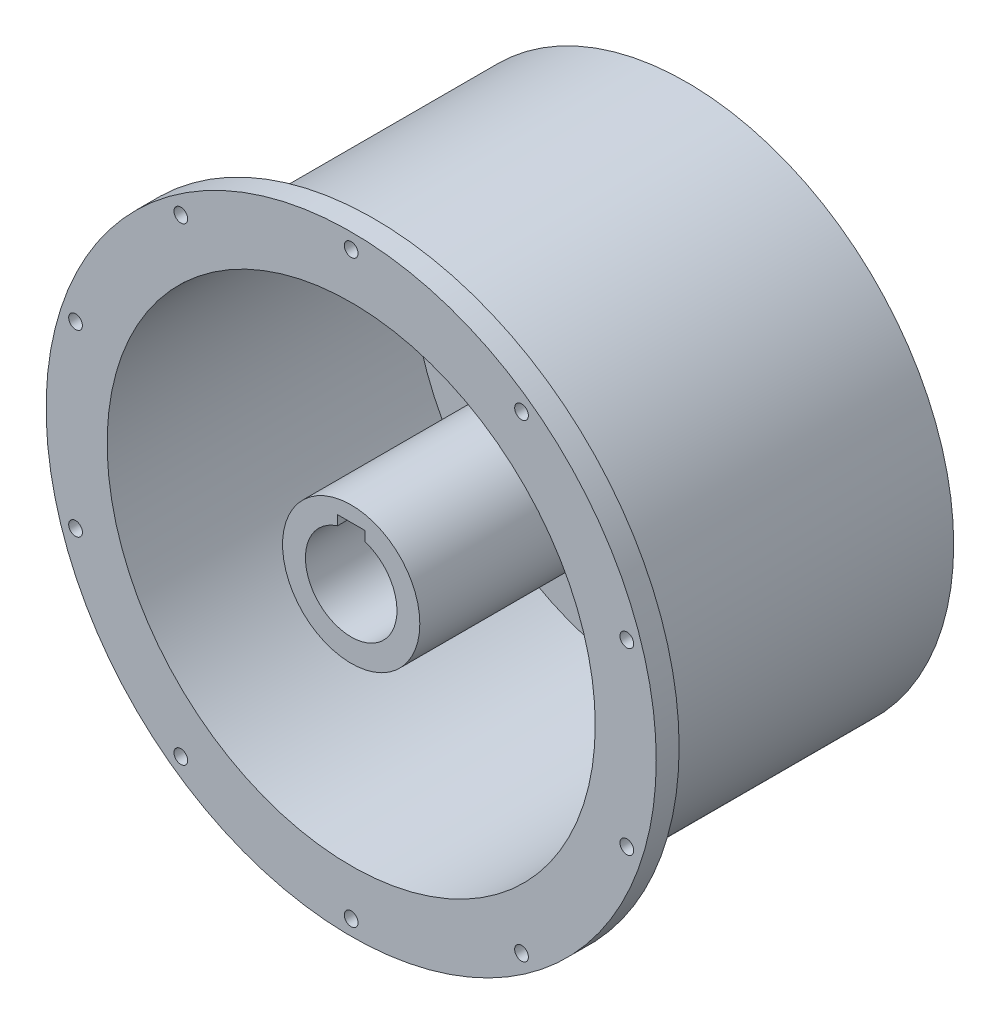
SolidWorks part; units mm, degrees
ref_plane "Front Plane" through (0, 0, 0) normal (0, 0, 1) x (1, 0, 0)
ref_plane "Top Plane" through (0, 0, 0) normal (0, 1, 0) x (1, 0, 0)
ref_plane "Right Plane" through (0, 0, 0) normal (1, 0, 0) x (0, 0, -1)
sketch "Sketch1" plane through (0, 0, 0) normal (0, 0, 1) x (1, 0, 0)
  circle A0 centre (0, 0) radius 30
  circle A1 centre (0, 0) radius 175
  dimension "D1" = 60
  dimension "D2" = 350
extrude "Boss-Extrude1" add sketch "Sketch1" along normal blind 220
sketch "Sketch2" plane through (0, 0, 220) normal (0, 0, 1) x (1, 0, 0)
  circle A0 centre (0, 0) radius 200
  circle A1 centre (0, 190) radius 4.5
  circle A2 centre (111.6792, 153.7132) radius 4.5
  circle A3 centre (180.7007, 58.7132) radius 4.5
  circle A4 centre (180.7007, -58.7132) radius 4.5
  circle A5 centre (111.6792, -153.7132) radius 4.5
  circle A6 centre (0, -190) radius 4.5
  circle A7 centre (-111.6792, -153.7132) radius 4.5
  circle A8 centre (-180.7007, -58.7132) radius 4.5
  circle A9 centre (-180.7007, 58.7132) radius 4.5
  circle A10 centre (-111.6792, 153.7132) radius 4.5
  circle A11 centre (0, 0) radius 30 construction
  circle A12 centre (0, 0) radius 30
  point P25 (0, 0)
  dimension "D1" = 400
  dimension "D2" = 9
  dimension "D3" = 190
  dimension "D4" = 10
extrude "Boss-Extrude2" add sketch "Sketch2" against normal blind 15
sketch "Sketch3" plane through (0, 0, 220) normal (0, 0, 1) x (1, 0, 0)
  circle A0 centre (0, 0) radius 45
  circle A1 centre (0, 0) radius 160
  dimension "D1" = 90
  dimension "D2" = 320
extrude "Cut-Extrude1" cut sketch "Sketch3" against normal blind 200
sketch "Sketch4" plane through (0, 0, 0) normal (0, 0, -1) x (-1, 0, 0)
  circle A0 centre (0, 0) radius 30 construction
  circle A1 centre (0, 0) radius 30
extrude "Boss-Extrude3" add sketch "Sketch4" against normal blind 20
sketch "Sketch7" plane through (0, 0, 220) normal (0, 0, 1) x (1, 0, 0)
  line L1 (-9, 35) -> (9, 35)
  line L2 (-9, 35) -> (-9, 14.7881)
  line L3 (-9, 14.7881) -> (9, 14.7881)
  line L4 (9, 35) -> (9, 14.7881)
  dimension "D1" = 18
  dimension "D2" = 9
  dimension "D3" = 35
extrude "Cut-Extrude2" cut sketch "Sketch7" against normal blind 200
